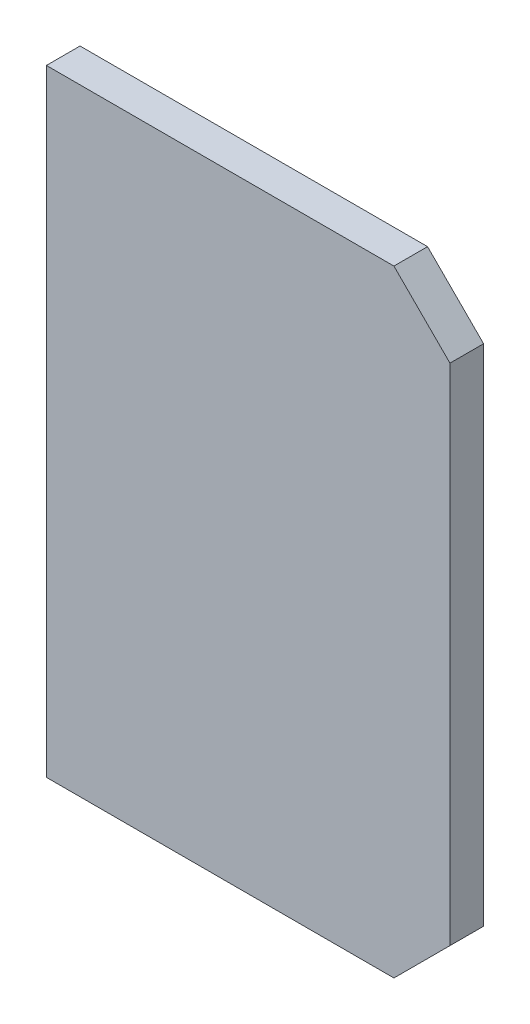
from build123d import *

# Parameters (mm, degrees)
SKETCH_1_W      = 36
SKETCH_1_H      = 55
EXTRUDE_1_DEPTH = 3
CHAMFER_1_SIZE  = 5


with BuildPart() as part:
    # 草图1 → 凸台-拉伸1 (new body)
    with BuildSketch(Plane.XY):
        with Locations((18, 27.5)):
            Rectangle(SKETCH_1_W, SKETCH_1_H)
    extrude(amount=EXTRUDE_1_DEPTH)

    # 倒角1
    chamfer_1_edges = [part.edges().sort_by_distance(p)[0] for p in [
        (36, 55, 1.5),
        (36, 0, 1.5),
    ]]
    chamfer(chamfer_1_edges, length=CHAMFER_1_SIZE)


solid = part.part
